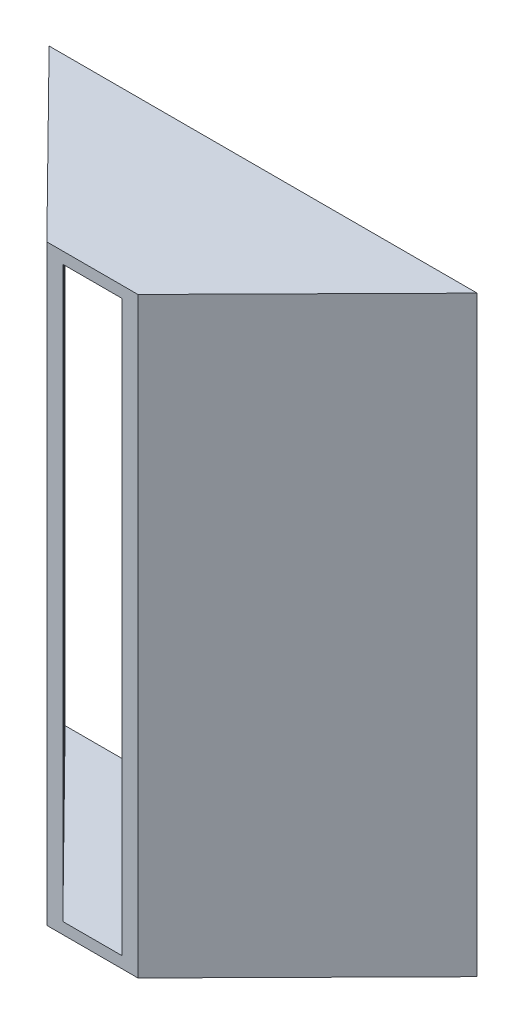
SolidWorks part; units mm, degrees
ref_plane "Front" through (0, 0, 0) normal (0, 0, 1) x (1, 0, 0)
ref_plane "Top" through (0, 0, 0) normal (0, 1, 0) x (1, 0, 0)
ref_plane "Right" through (0, 0, 0) normal (1, 0, 0) x (0, 0, -1)
sketch "Sketch1" plane through (0, 0, 0) normal (0, 1, 0) x (1, 0, 0)
  line L0 (0, 0) -> (40, 0)
  line L1 (40, 0) -> (188, 150)
  line L2 (188, 150) -> (0, 150)
  line L3 (0, 0) -> (0, 150)
  dimension "D1" = 40
  dimension "D2" = 150
  dimension "D3" = 188
extrude "Boss-Extrude1" add sketch "Sketch1" along normal blind 520
mirror "Mirror1" about plane through (0, 520, 0) normal (1, 0, 0) of "Boss-Extrude1"
shell "Shell1" thickness 10
